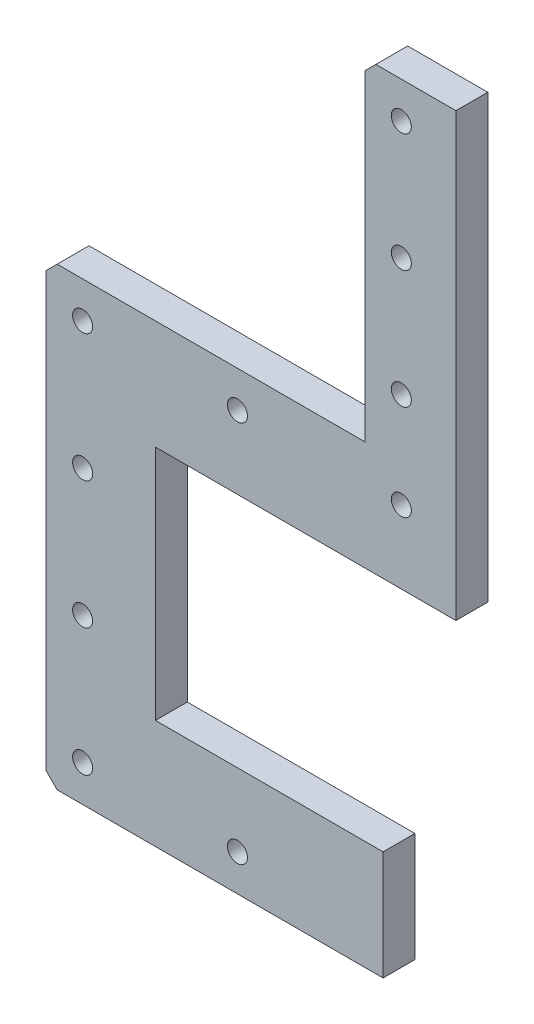
from build123d import *

# Parameters (mm, degrees)
EXTRUDE_1_DEPTH          = 35
CHAMFER_1_SIZE           = 12
CUT_EXTRUDE_1_DEPTH      = 976.679250574
CUT_EXTRUDE_1_DEPTH_BACK = 976.679250574
SKETCH_2_R               = 11


with BuildPart() as part:
    # 草图1 → 凸台-拉伸1 (new body)
    with BuildSketch(Plane.XY):
        Polygon((0, 0), (0, -485), (-330, -485), (-330, -745), (-80, -745), (-80, -865), (-450, -865), (-450, -365), (-100, -365), (-100, 0), align=None)
    extrude(amount=EXTRUDE_1_DEPTH)

    # 倒角1
    chamfer_1_edges = [part.edges().sort_by_distance(p)[0] for p in [
        (-100, 0, 17.5),
        (-450, -865, 17.5),
        (-450, -365, 17.5),
    ]]
    chamfer(chamfer_1_edges, length=CHAMFER_1_SIZE)

    # 草图2 → 切除-拉伸1 (cut, two sides: drawn at the far end of the back side and taken through both)
    with BuildSketch(Plane.XY.offset(35).offset(-CUT_EXTRUDE_1_DEPTH_BACK)):
        with Locations((-60, -40)):
            Circle(SKETCH_2_R)
        with Locations((-60, -170)):
            Circle(SKETCH_2_R)
        with Locations((-60, -300)):
            Circle(SKETCH_2_R)
        with Locations((-60, -405)):
            Circle(SKETCH_2_R)
        with Locations((-240, -405)):
            Circle(SKETCH_2_R)
        with Locations((-410, -405)):
            Circle(SKETCH_2_R)
        with Locations((-410, -545)):
            Circle(SKETCH_2_R)
        with Locations((-410, -685)):
            Circle(SKETCH_2_R)
        with Locations((-410, -825)):
            Circle(SKETCH_2_R)
        with Locations((-240, -825)):
            Circle(SKETCH_2_R)
    extrude(amount=CUT_EXTRUDE_1_DEPTH + CUT_EXTRUDE_1_DEPTH_BACK, mode=Mode.SUBTRACT)


solid = part.part
